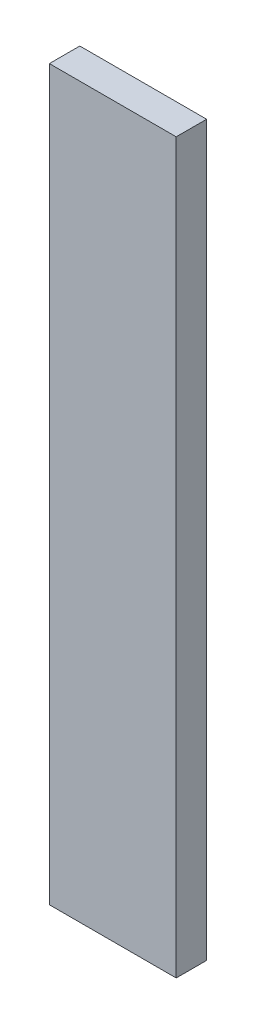
SolidWorks part; units mm, degrees
material "Q235"
ref_plane "Front Plane" through (0, 0, 0) normal (0, 0, 1) x (1, 0, 0)
ref_plane "Top Plane" through (0, 0, 0) normal (0, 1, 0) x (1, 0, 0)
ref_plane "Right Plane" through (0, 0, 0) normal (1, 0, 0) x (0, 0, -1)
sketch "Sketch1" plane through (0, 0, 0) normal (0, 0, 1) x (1, 0, 0)
  line L1 (0, 0) -> (125, 0)
  line L2 (0, 0) -> (0, 718)
  line L3 (0, 718) -> (125, 718)
  line L4 (125, 0) -> (125, 718)
  dimension "D1" = 718
  dimension "D2" = 125
extrude "Boss-Extrude1" add sketch "Sketch1" along normal blind 30
